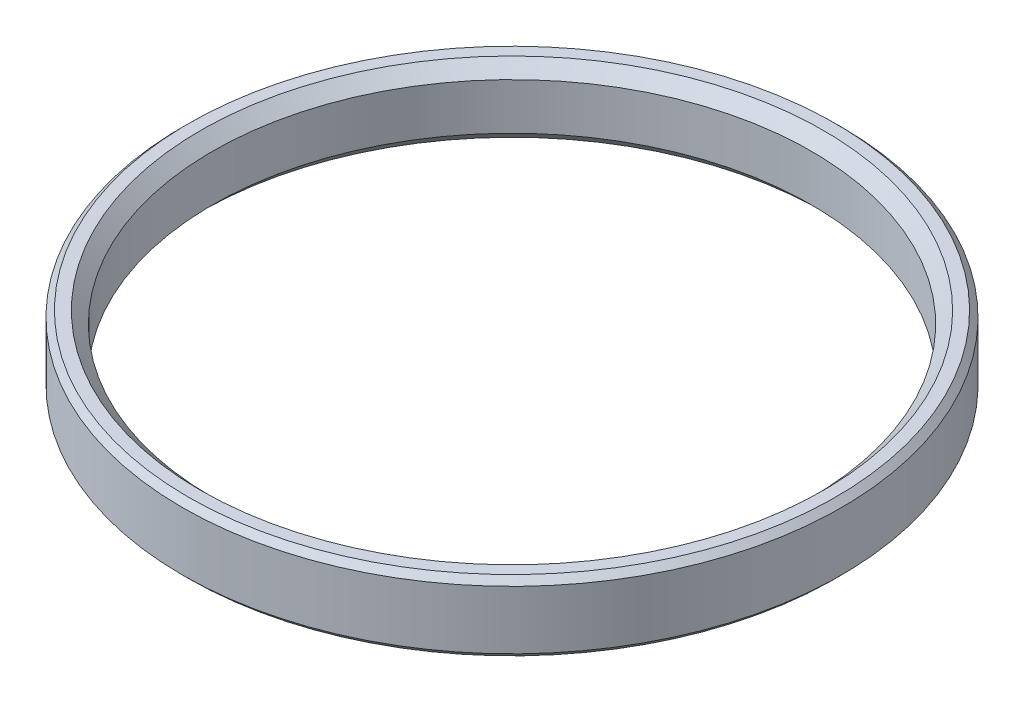
from build123d import *

# Parameters (mm, degrees)
SKETCH1_R           = 55
SKETCH1_R_2         = 50
BOSS_EXTRUDE1_DEPTH = 11.75
CHAMFER1_SIZE       = 1
CHAMFER2_SIZE       = 2


with BuildPart() as part:
    # Sketch1 → Boss-Extrude1 (new body)
    with BuildSketch(Plane(origin=(0, 0, 0), x_dir=(1, 0, 0), z_dir=(0, 1, 0))):
        with Locations(Location((0, 0, 0), (0, 0, 270))):
            Circle(SKETCH1_R)
        with Locations(Location((0, 0, 0), (0, 0, 270))):
            Circle(SKETCH1_R_2, mode=Mode.SUBTRACT)
    extrude(amount=BOSS_EXTRUDE1_DEPTH)

    # Chamfer1
    chamfer1_edges = [part.edges().sort_by_distance(p)[0] for p in [
        (0, 0, -55),
        (0, 11.75, -55),
    ]]
    chamfer(chamfer1_edges, length=CHAMFER1_SIZE)

    # Chamfer2
    chamfer2_edges = [part.edges().sort_by_distance(p)[0] for p in [
        (0, 0, -50),
        (0, 11.75, -50),
    ]]
    chamfer(chamfer2_edges, length=CHAMFER2_SIZE)


solid = part.part
